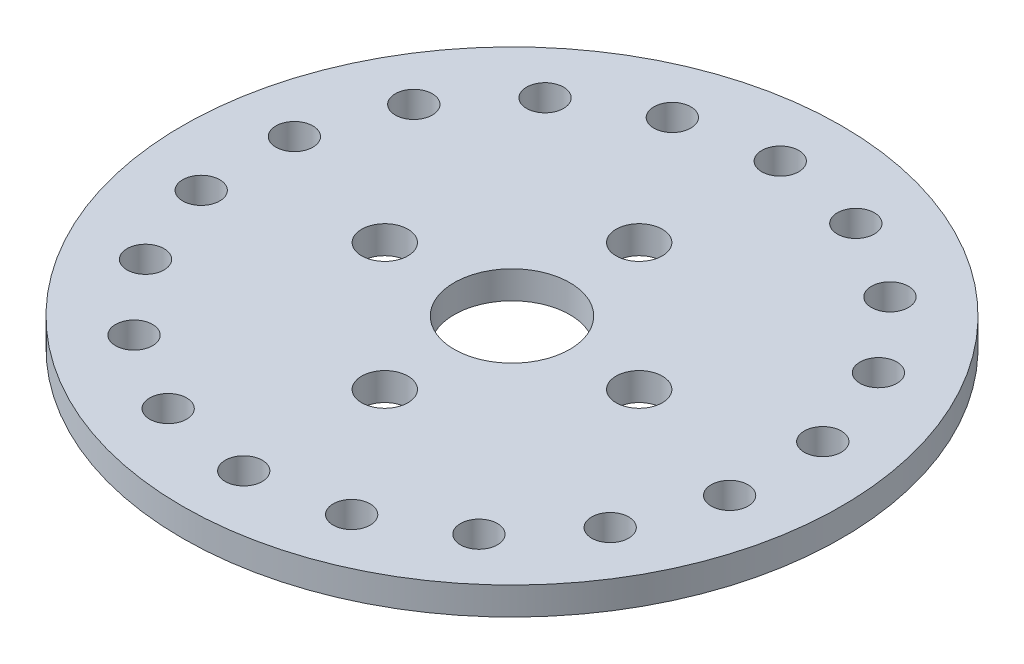
from build123d import *

# Parameters (mm, degrees)
SKETCH1_R                  = 142.5
SKETCH1_R_2                = 25
BOSS_EXTRUDE1_DEPTH        = 6
F_20_0_20_DIAMETER_HOLE1_D = 20
F_16_0_16_DIAMETER_HOLE1_D = 16


with BuildPart() as part:
    # Sketch1 → Boss-Extrude1 (new, symmetric)
    with BuildSketch(Plane(origin=(0, 0, 0), x_dir=(1, 0, 0), z_dir=(0, 1, 0))):
        with Locations(Location((0, 0, 0), (0, 0, 270))):
            Circle(SKETCH1_R)
        with Locations(Location((0, 0, 0), (0, 0, 270))):
            Circle(SKETCH1_R_2, mode=Mode.SUBTRACT)
    extrude(amount=BOSS_EXTRUDE1_DEPTH, both=True)

    # Ø20.0 (20) Diameter Hole1 (through all)
    with Locations(Plane(origin=(0, 6, 0), x_dir=(1, 0, 0), z_dir=(0, 1, 0))):
        with Locations((0, 55), (55, 0), (0, -55), (-55, 0)):
            Hole(F_20_0_20_DIAMETER_HOLE1_D / 2)

    # Ø16.0 (16) Diameter Hole1 (through all)
    with Locations(Plane(origin=(0, 6, 0), x_dir=(1, 0, 0), z_dir=(0, 1, 0))):
        with Locations((0, 116), (39.674336626, 109.004344011), (74.563362724, 88.861155402), (100.458946839, 58), (114.237699349, 20.143188609), (114.237699349, -20.143188609), (100.458946839, -58), (74.563362724, -88.861155402), (39.674336626, -109.004344011), (0, -116), (-39.674336626, -109.004344011), (-74.563362724, -88.861155402), (-100.458946839, -58), (-114.237699349, -20.143188609), (-114.237699349, 20.143188609), (-100.458946839, 58), (-74.563362724, 88.861155402), (-39.674336626, 109.004344011)):
            Hole(F_16_0_16_DIAMETER_HOLE1_D / 2)


solid = part.part
